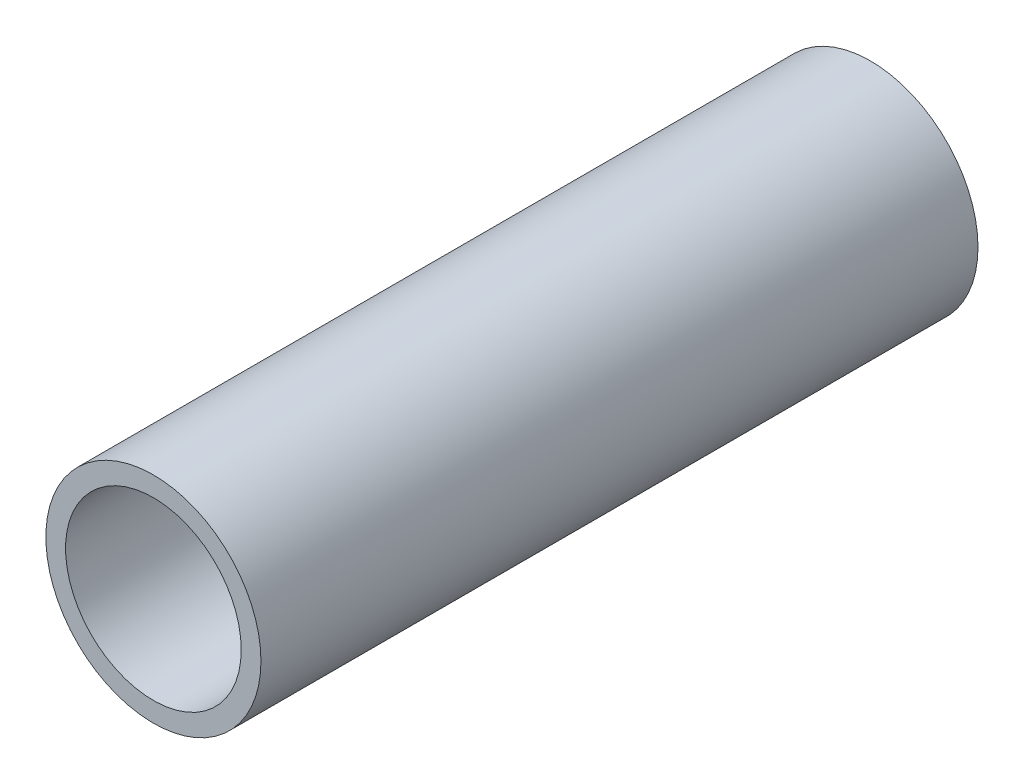
from build123d import *

# Parameters (mm, degrees)
SKETCH_1_R      = 3
SKETCH_1_R_2    = 2.45
EXTRUDE_1_DEPTH = 20


with BuildPart() as part:
    # 草图1 → 凸台-拉伸1 (new body)
    with BuildSketch(Plane.XY):
        Circle(SKETCH_1_R)
        Circle(SKETCH_1_R_2, mode=Mode.SUBTRACT)
    extrude(amount=-EXTRUDE_1_DEPTH)


solid = part.part
